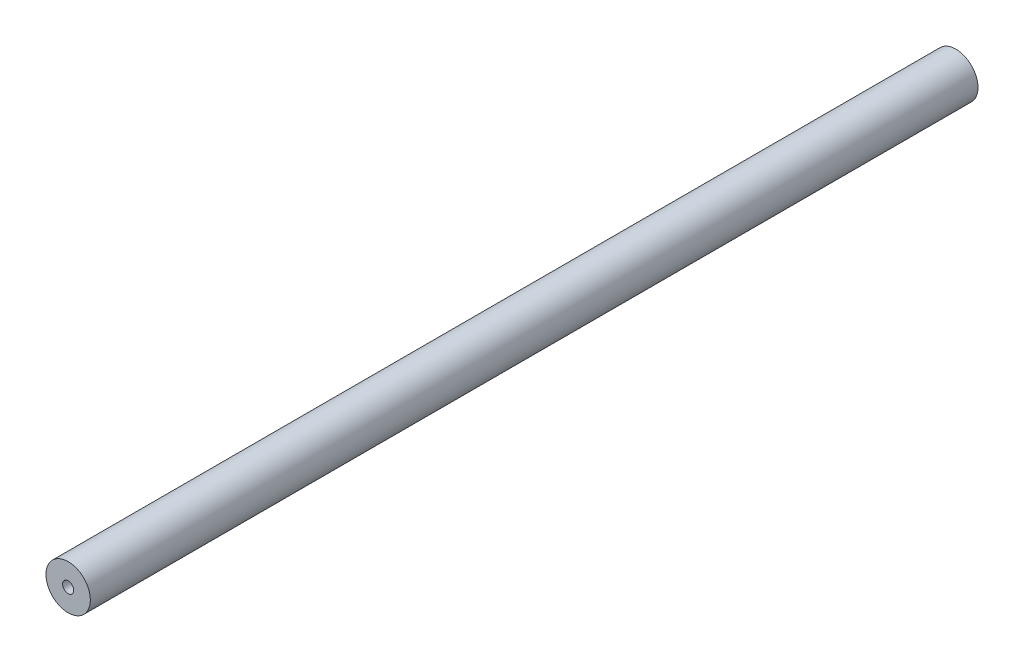
SolidWorks part; units mm, degrees
ref_plane "Front Plane" through (0, 0, 0) normal (0, 0, 1) x (1, 0, 0)
ref_plane "Top Plane" through (0, 0, 0) normal (0, 1, 0) x (1, 0, 0)
ref_plane "Right Plane" through (0, 0, 0) normal (1, 0, 0) x (0, 0, -1)
sketch "Sketch1" plane through (0, 0, 0) normal (0, 0, 1) x (1, 0, 0)
  circle A0 centre (0, 0) radius 10
  dimension "D1" = 20
extrude "Boss-Extrude1" add sketch "Sketch1" along normal blind 400
hole_wizard "M6 Tapped Hole1" positions "Sketch2" profile "Sketch3" tap size "M6" standard "GB"
sketch "Sketch2" plane through (0, 0, 400) normal (0, 0, 1) x (1, 0, 0)
  point P0 (0, 0)
sketch "Sketch3" plane through (0, 0, 400) normal (1, 0, 0) x (0, -1, 0)
  line L0 (0, 0) -> (0, 16.5022)
  line L1 (0, 16.5022) -> (2.5, 15)
  line L2 (2.5, 15) -> (2.5, 0)
  line L5 (2.5, 0) -> (0, 0)
  line L10 (0, 16.5022) -> (-2.5, 15) construction
  line L11 (0, -6.35) -> (0, 107.95) construction
  dimension "螺纹孔钻头直径" = 5
  dimension "螺纹孔钻头深度" = 15
  dimension "导头角度" = 118
cosmetic thread "Hole Thread1" parameters "D1"=12, "D2"=6
hole_wizard "M6 Tapped Hole2" positions "Sketch4" profile "Sketch5" tap size "M6" standard "GB"
sketch "Sketch4" plane through (0, 0, 0) normal (0, 0, -1) x (-1, 0, 0)
  point P0 (0, 0)
sketch "Sketch5" plane through (0, 0, 0) normal (1, 0, 0) x (0, 1, 0)
  line L0 (0, 0) -> (0, 16.5022)
  line L1 (0, 16.5022) -> (2.5, 15)
  line L2 (2.5, 15) -> (2.5, 0)
  line L5 (2.5, 0) -> (0, 0)
  line L10 (0, 16.5022) -> (-2.5, 15) construction
  line L11 (0, -6.35) -> (0, 107.95) construction
  dimension "螺纹孔钻头直径" = 5
  dimension "螺纹孔钻头深度" = 15
  dimension "导头角度" = 118
cosmetic thread "Hole Thread2" parameters "D1"=12, "D2"=6
